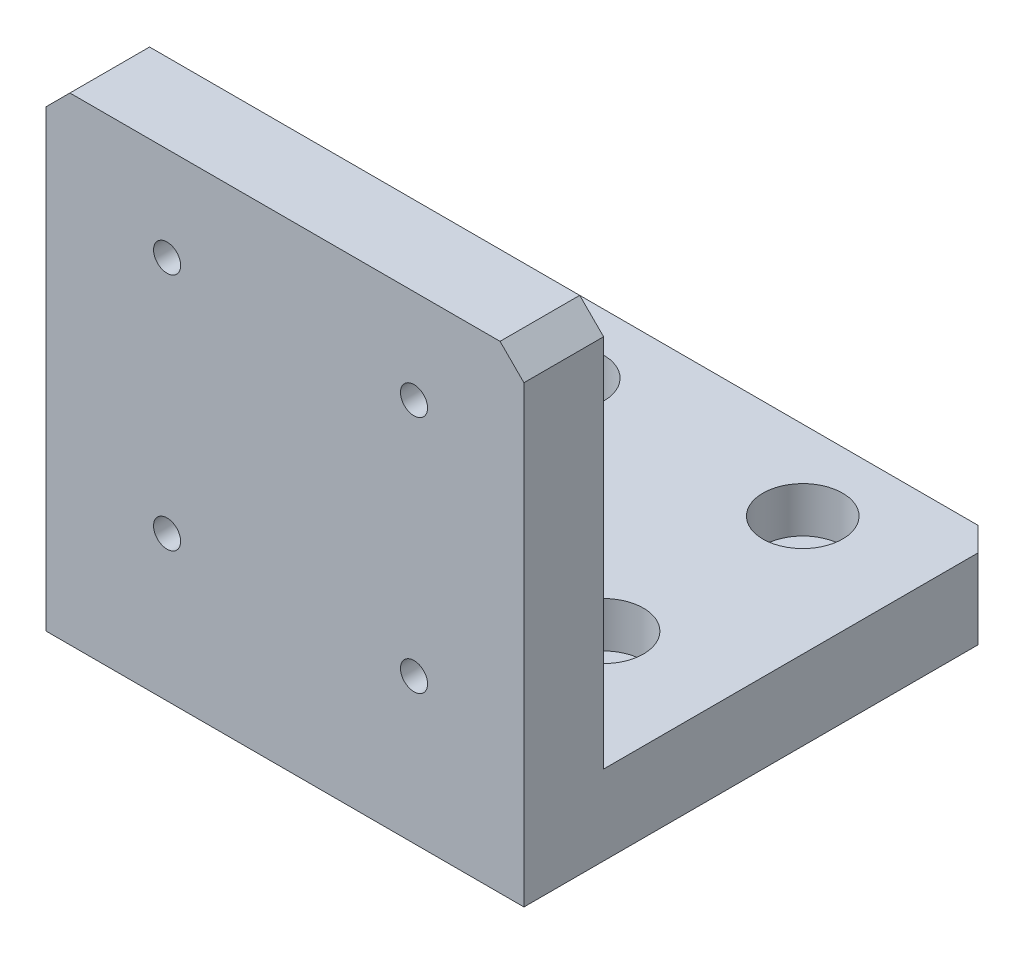
from build123d import *

# Parameters (mm, degrees)
SKETCH_1_W                = 60
SKETCH_1_H                = 60
EXTRUDE_1_DEPTH           = 10
SKETCH_2_W                = 60
SKETCH_2_H                = 10
EXTRUDE_2_DEPTH           = 50
CHAMFER_1_SIZE            = 3
HOLE_WIZARD_1_D           = 5.5
HOLE_WIZARD_1_DEPTH       = 15
HOLE_WIZARD_1_CBORE_D     = 10
HOLE_WIZARD_1_CBORE_DEPTH = 5.7
HOLE_WIZARD_1_TIP         = 1.652366702
HOLE_WIZARD_2_D           = 3.4
HOLE_WIZARD_2_DEPTH       = 15
HOLE_WIZARD_2_CBORE_D     = 6
HOLE_WIZARD_2_CBORE_DEPTH = 3.4
HOLE_WIZARD_2_TIP         = 1.021463052


with BuildPart() as part:
    # 草图1 → 凸台-拉伸1 (new body)
    with BuildSketch(Plane(origin=(0, 0, 0), x_dir=(1, 0, 0), z_dir=(0, 1, 0))):
        Rectangle(SKETCH_1_W, SKETCH_1_H)
    extrude(amount=EXTRUDE_1_DEPTH)

    # 草图2 → 凸台-拉伸2 (add)
    with BuildSketch(Plane(origin=(0, 10, 0), x_dir=(1, 0, 0), z_dir=(0, 1, 0))):
        with Locations((0, -25)):
            Rectangle(SKETCH_2_W, SKETCH_2_H)
    extrude(amount=EXTRUDE_2_DEPTH)

    # 倒角1
    chamfer_1_edges = [part.edges().sort_by_distance(p)[0] for p in [
        (-30, 60, 25),
        (30, 60, 25),
        (-30, 5, -30),
        (30, 5, -30),
    ]]
    chamfer(chamfer_1_edges, length=CHAMFER_1_SIZE)

    # 打孔尺寸(%根据)内六角圆柱头螺钉的类型1
    with Locations(Plane(origin=(0, 10, 0), x_dir=(1, 0, 0), z_dir=(0, 1, 0))):
        with Locations((-15, 20), (15, 20), (-15, -5), (15, -5)):
            CounterBoreHole(HOLE_WIZARD_1_D / 2, HOLE_WIZARD_1_CBORE_D / 2, HOLE_WIZARD_1_CBORE_DEPTH, depth=HOLE_WIZARD_1_DEPTH)
            with Locations((0, 0, -(HOLE_WIZARD_1_DEPTH + HOLE_WIZARD_1_TIP / 2))):  # 118° drill point
                Cone(0, HOLE_WIZARD_1_D / 2, HOLE_WIZARD_1_TIP, mode=Mode.SUBTRACT)

    # 打孔尺寸(%根据)内六角圆柱头螺钉的类型2
    with Locations(Plane(origin=(0, 0, 20), x_dir=(-1, 0, 0), z_dir=(0, 0, -1))):
        with Locations((-16.2, 48.2), (14.8, 48.2), (-16.2, 18.2), (14.8, 18.2)):
            CounterBoreHole(HOLE_WIZARD_2_D / 2, HOLE_WIZARD_2_CBORE_D / 2, HOLE_WIZARD_2_CBORE_DEPTH, depth=HOLE_WIZARD_2_DEPTH)
            with Locations((0, 0, -(HOLE_WIZARD_2_DEPTH + HOLE_WIZARD_2_TIP / 2))):  # 118° drill point
                Cone(0, HOLE_WIZARD_2_D / 2, HOLE_WIZARD_2_TIP, mode=Mode.SUBTRACT)


solid = part.part
